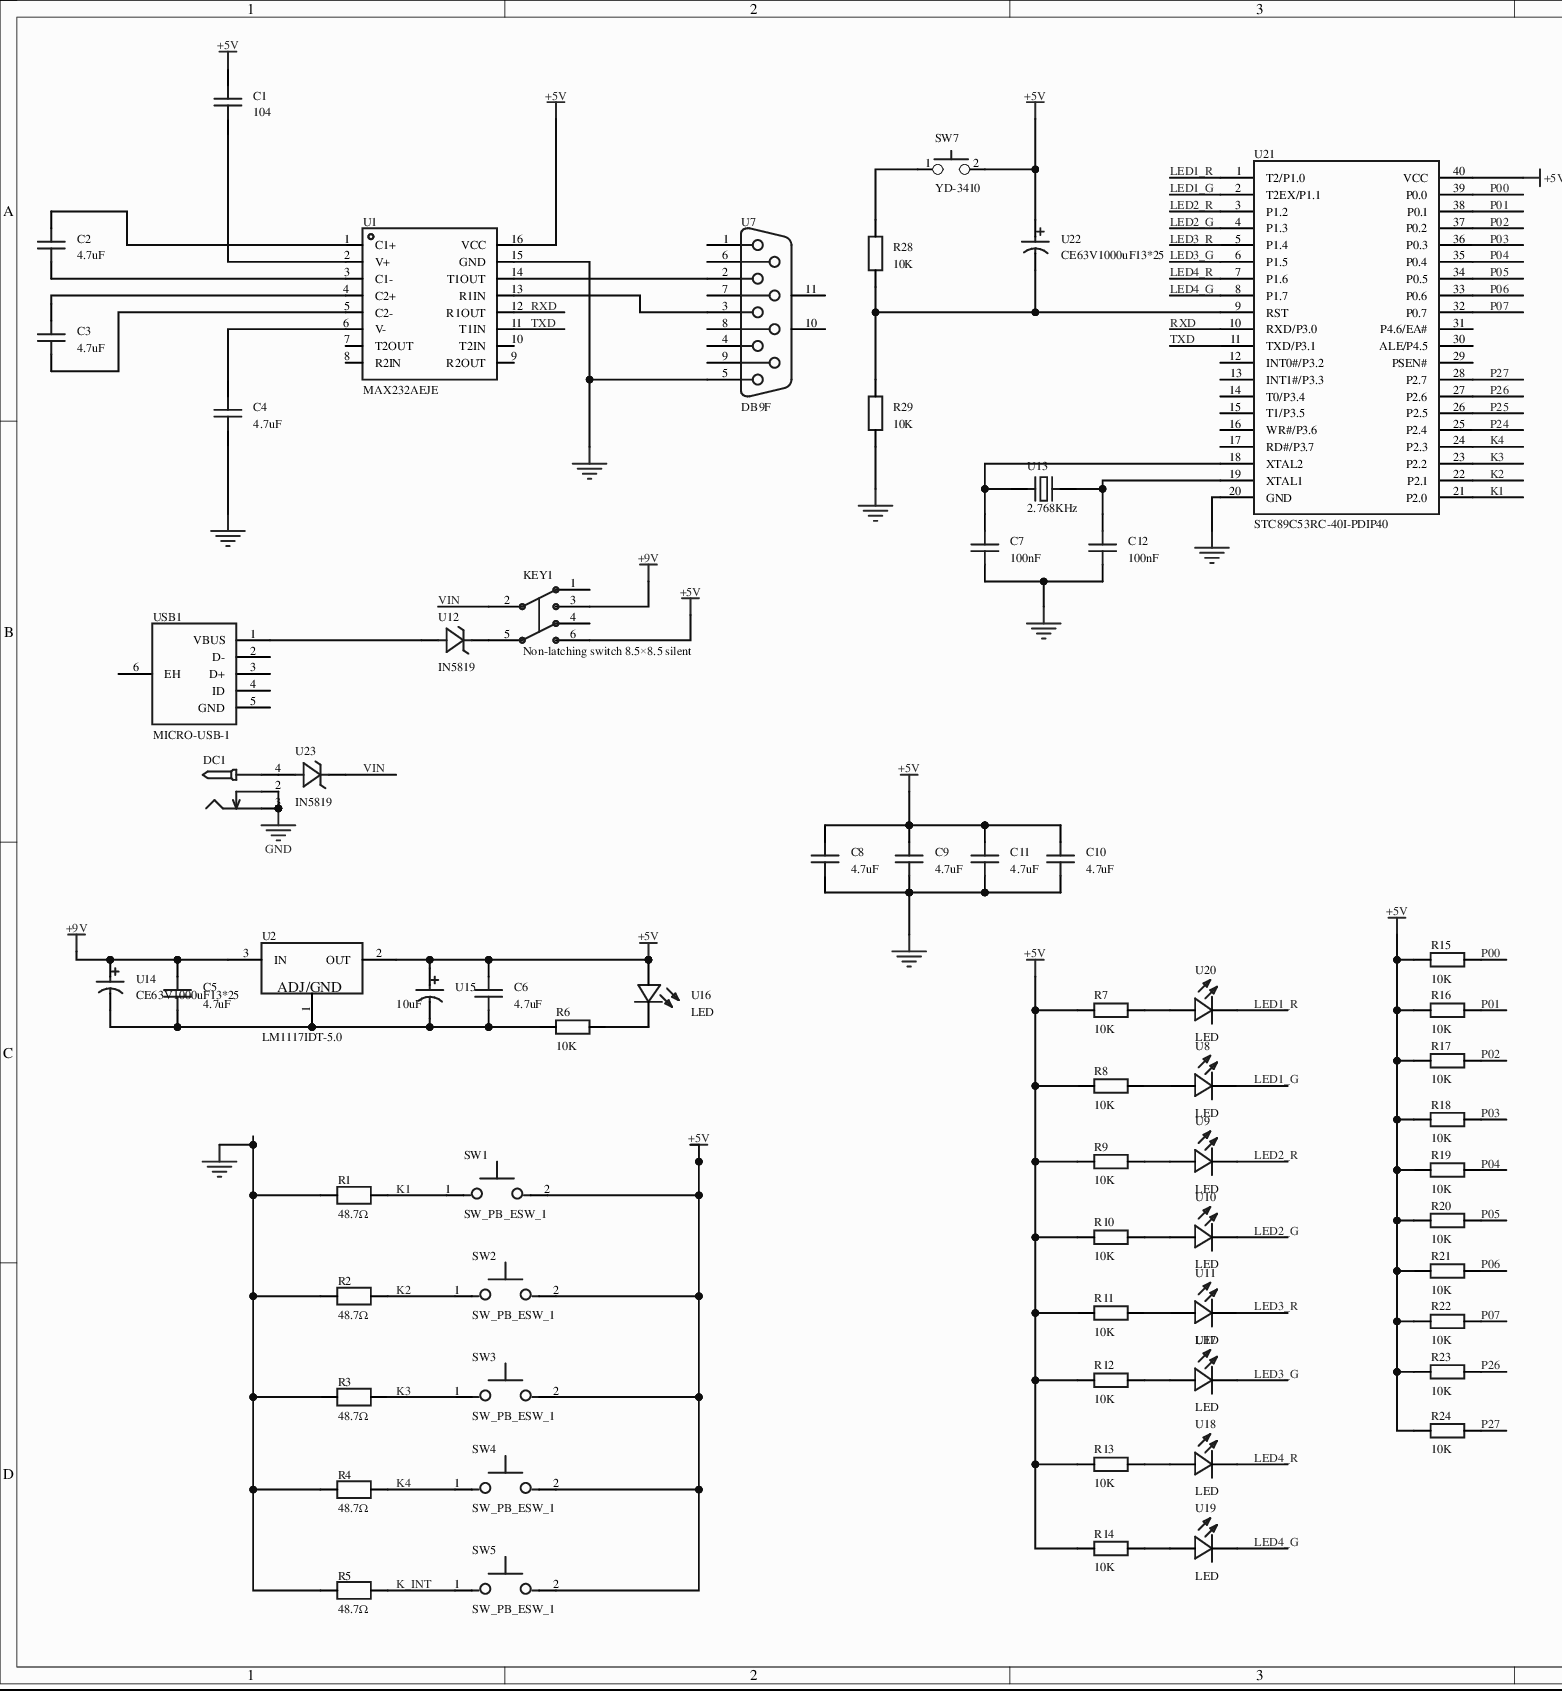
[diagram p0: MISC51895-3.schdoc, left]
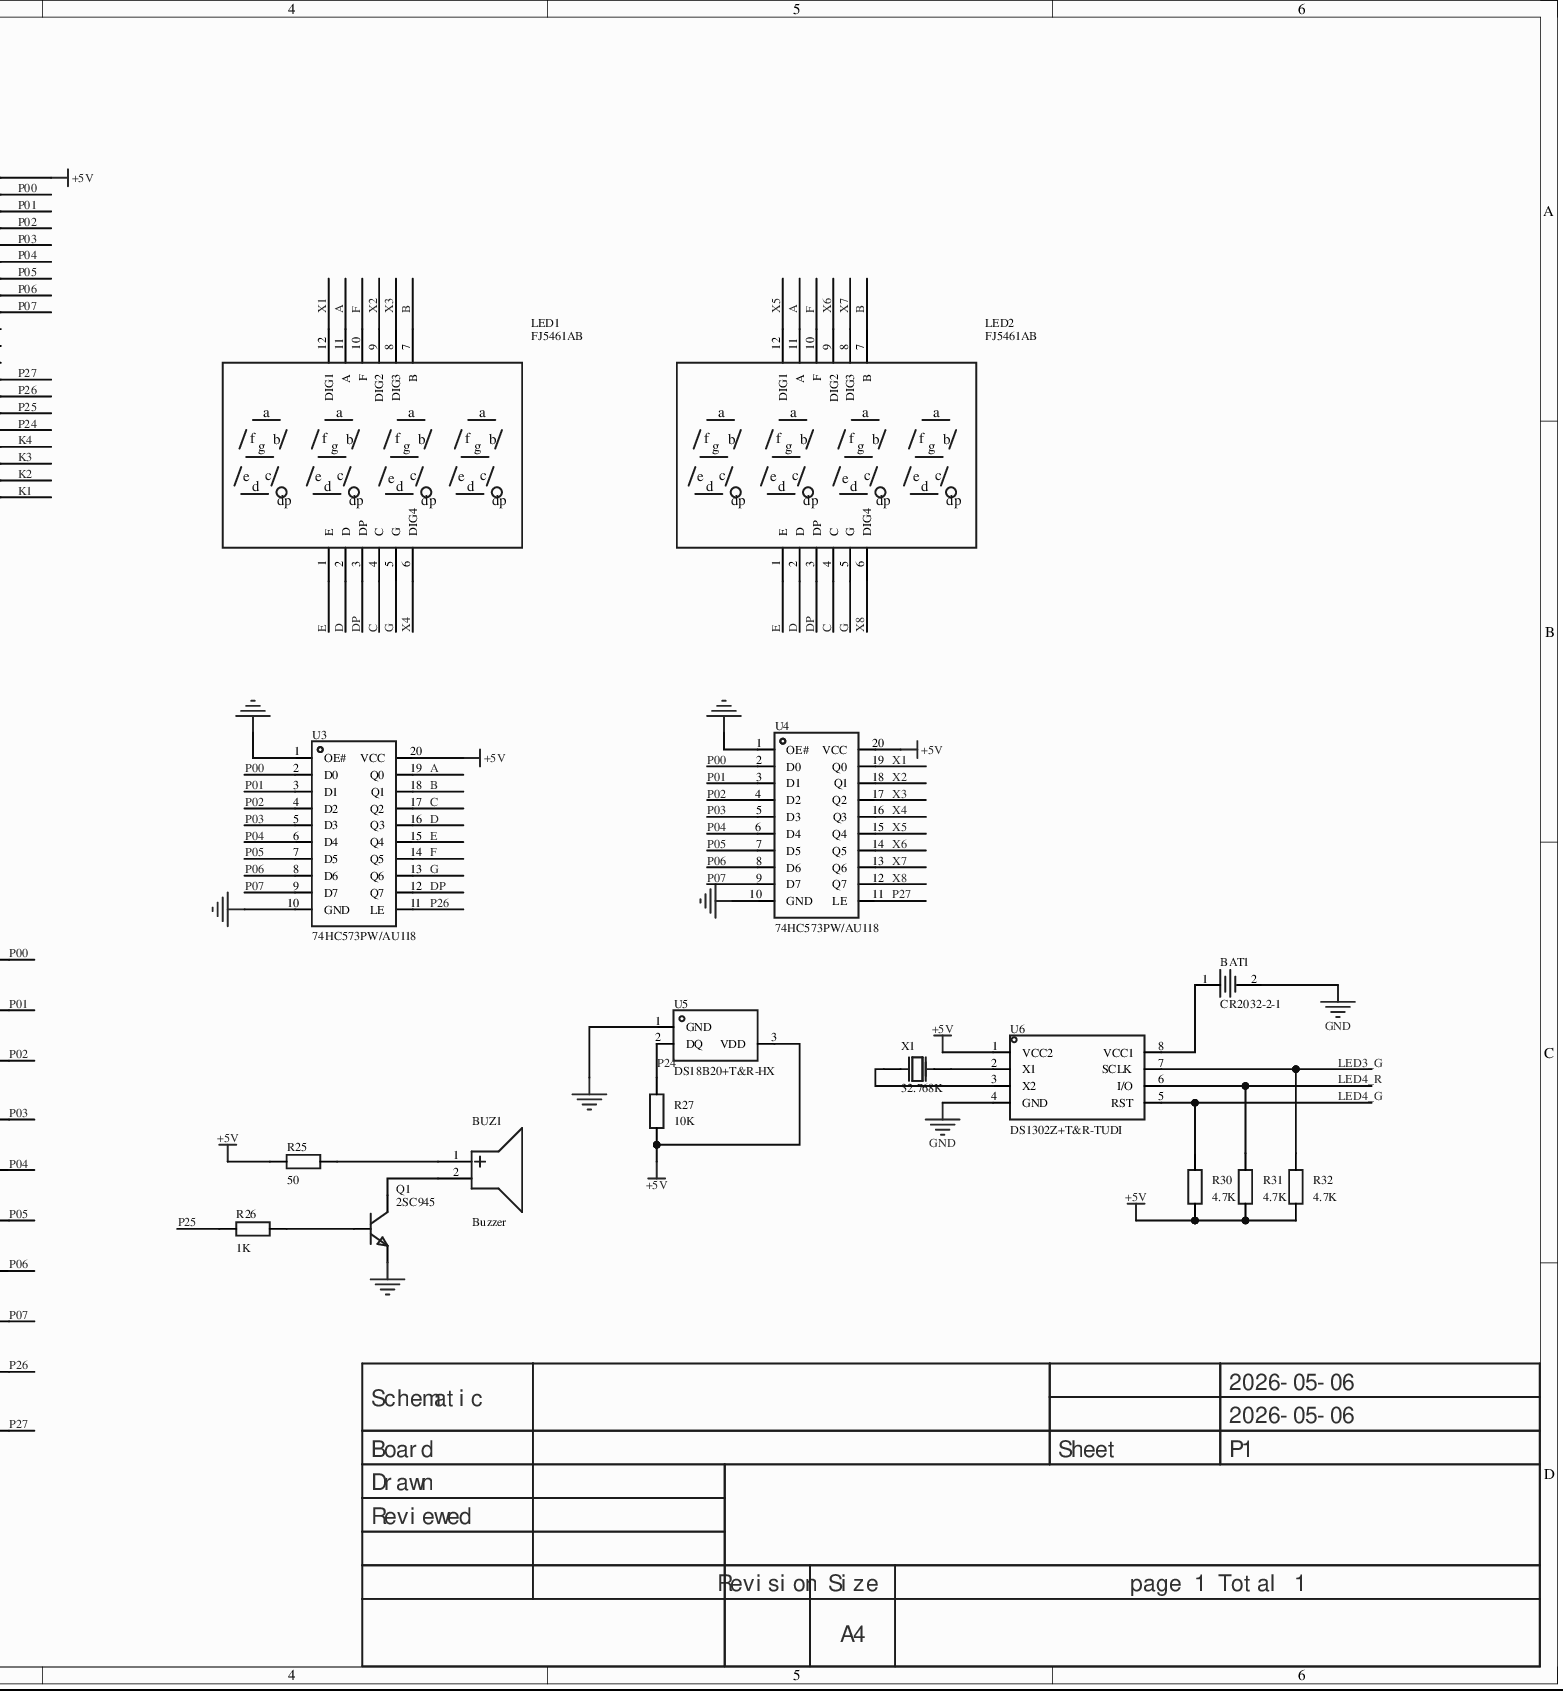
[diagram p1: MISC51895-3.schdoc, right]
# Altium project MISC51895-2.PrjPcb
1 sheet, 82 parts. Net scope: global (net labels, ports and power ports of the same name join across sheets).
Board file: MISC51895.pcbdoc

## Sheet MISC51895-3.schdoc
size 457 x 254 mm; Version: V1.0; @Project Name: MISC51895; @Update Date: 2026-05-06; @Create Date: 2026-05-06; @Board Name: MISC51895; @Create Time: 08:32:17; @Page Count: 1; @Page No: 1; @Schematic Name: MISC51895; @Update Time: 08:32:17; Size: A4

### Parts
BAT1  CR2032-2-1  [BAT-TH_CR2032-2-1]
BUZ1  Buzzer  [BUZ-TH_BD9.0-P5.00-D0.6-FD]
C1  104  [C0603]
C2  4.7uF  [C0603]
C3  4.7uF  [C0603]
C4  4.7uF  [C0603]
C5  4.7uF  [C0603]
C6  4.7uF  [C0603]
C7  100nF  [C0603]
C8  4.7uF  [C0603]
C9  4.7uF  [C0603]
C10  4.7uF  [C0603]
C11  4.7uF  [C0603]
C12  100nF  [C0603]
DC1  (no value)  [DC-2.0]
KEY1  Non-latching switch 8.5×8.5 silent  [SW-TH_6P-L8.5-W8.5-P2.54]
LED1  FJ5461AB  [LED-SEG-TH_12P-L50.4-W19.0-P2.54-S15.24-BL]
LED2  FJ5461AB  [LED-SEG-TH_12P-L50.4-W19.0-P2.54-S15.24-BL]
Q1  2SC945  [TO-92-3_L4.9-W3.7-P1.27-L]
R1  48.7Ω  [R0603]
R2  48.7Ω  [R0603]
R3  48.7Ω  [R0603]
R4  48.7Ω  [R0603]
R5  48.7Ω  [R0603]
R6  10K  [R0603]
R7  10K  [R0603]
R8  10K  [R0603]
R9  10K  [R0603]
R10  10K  [R0603]
R11  10K  [R0603]
R12  10K  [R0603]
R13  10K  [R0603]
R14  10K  [R0603]
R15  10K  [R0603]
R16  10K  [R0603]
R17  10K  [R0603]
R18  10K  [R0603]
R19  10K  [R0603]
R20  10K  [R0603]
R21  10K  [R0603]
R22  10K  [R0603]
R23  10K  [R0603]
R24  10K  [R0603]
R25  50  [R0603]
R26  1K  [R0603]
R27  10K  [R0603]
R28  10K  [R0603]
R29  10K  [R0603]
R30  4.7K  [R0603]
R31  4.7K  [R0603]
R32  4.7K  [R0603]
SW1  SW_PB_ESW_1  [KEY-SMD_L6.1-W3.8-LS8.0]
SW2  SW_PB_ESW_1  [KEY-SMD_L6.1-W3.8-LS8.0]
SW3  SW_PB_ESW_1  [KEY-SMD_L6.1-W3.8-LS8.0]
SW4  SW_PB_ESW_1  [KEY-SMD_L6.1-W3.8-LS8.0]
SW5  SW_PB_ESW_1  [KEY-SMD_L6.1-W3.8-LS8.0]
SW7  YD-3410  [SW-SMD_L3.9-W2.9-LS4.8-EH-A]
U1  MAX232AEJE  [PDIP-16_L19.3-W6.5-P2.54-LS7.6-BL]
U2  LM1117IDT-5.0  [TO-252-2_L6.6-W6.1-P4.57-LS9.7-BR-CW]
U3  74HC573PW/AU118  [TSSOP-20_L6.5-W4.4-P0.65-LS6.4-BL]
U4  74HC573PW/AU118  [TSSOP-20_L6.5-W4.4-P0.65-LS6.4-BL]
U5  DS18B20+T&R-HX  [TO-92-3_L5.1-W4.1-P1.27-L-1]
U6  DS1302Z+T&R-TUDI  [SOIC-8_L4.9-W3.9-P1.27-LS6.0-BL]
U7  DB9F  [DB9-TH_DB9F_C9900018961]
U8  LED  [LED-TH_BD4.0-P2.54-FD_RED]
U9  LED  [LED-TH_BD4.0-P2.54-FD_RED]
U10  LED  [LED-TH_BD4.0-P2.54-FD_RED]
U11  LED  [LED-TH_BD4.0-P2.54-FD_RED]
U12  IN5819  [SOD-123_L2.7-W1.7-LS3.8-RD]
U13  2.768KHz  [CRYSTAL-SMD_L3.2-W1.5-1]
U14  CE63V1000uF13*25  [CAP-TH_BD13.0-P5.00-D0.6-FD]
U15  10uF  [CAP-TH_BD13.0-P5.00-D0.6-FD]
U16  LED  [LED-TH_BD4.0-P2.54-FD_RED]
U17  LED  [LED-TH_BD4.0-P2.54-FD_RED]
U18  LED  [LED-TH_BD4.0-P2.54-FD_RED]
U19  LED  [LED-TH_BD4.0-P2.54-FD_RED]
U20  LED  [LED-TH_BD4.0-P2.54-FD_RED]
U21  STC89C53RC-40I-PDIP40  [DIP-40_L52.0-W13.7-P2.54-LS15.2-BL]
U22  CE63V1000uF13*25  [CAP-TH_BD13.0-P5.00-D0.6-FD]
U23  IN5819  [SOD-123_L2.7-W1.7-LS3.8-RD]
USB1  MICRO-USB-1  [MICRO-USB-SMD_C9900008946]
X1  32.768K  [OSC-SMD_L2.0-W1.2]

### Nets
+5V: C1.2 C6.2 C8.2 C9.2 C10.2 C11.2 KEY1.6 R7.1 R8.1 R9.1 R10.1 R11.1 R12.1 R13.1 R14.1 R15.1 R16.1 R17.1 R18.1 R19.1 R20.1 R21.1 R22.1 R23.1 R24.1 R25.1 R27.1 R30.1 R31.1 R32.1 SW1.2 SW2.2 SW3.2 SW4.2 SW5.2 SW7.2 U1.16(VCC) U2.2(OUT) U3.20(VCC) U4.20(VCC) U5.3(VDD) U6.1(VCC2) U15.1 U16.1(+) U21.40(VCC) U22.1
+9V: C5.2 KEY1.3 U2.3(IN) U14.1
GND: BAT1.2 C4.1 C7.1 C8.1 C9.1 C10.1 C11.1 C12.1 DC1.2 DC1.3 Q1.1(E) R1.1 R2.1 R3.1 R4.1 R5.1 R29.1 U1.15(GND) U3.1(OE#) U3.10(GND) U4.1(OE#) U4.10(GND) U5.1(GND) U6.4(GND) U7.5 U21.20(GND)
A: LED1.11(A) LED2.11(A) U3.19(Q0)
B: LED1.7(B) LED2.7(B) U3.18(Q1)
C: LED1.4(C) LED2.4(C) U3.17(Q2)
D: LED1.2(D) LED2.2(D) U3.16(Q3)
DP: LED1.3(DP) LED2.3(DP) U3.12(Q7)
E: LED1.1(E) LED2.1(E) U3.15(Q4)
F: LED1.10(F) LED2.10(F) U3.14(Q5)
G: LED1.5(G) LED2.5(G) U3.13(Q6)
K1: R1.2 SW1.1 U21.21(P2.0)
K2: R2.2 SW2.1 U21.22(P2.1)
K3: R3.2 SW3.1 U21.23(P2.2)
K4: R4.2 SW4.1 U21.24(P2.3)
K_INT: R5.2 SW5.1
LED1_G: U8.2(-) U21.2(T2EX/P1.1)
LED1_R: U20.2(-) U21.1(T2/P1.0)
LED2_G: U10.2(-) U21.4(P1.3)
LED2_R: U9.2(-) U21.3(P1.2)
LED3_G: R32.2 U6.7(SCLK) U17.2(-) U21.6(P1.5)
LED3_R: U11.2(-) U21.5(P1.4)
LED4_G: R30.2 U6.5(RST) U19.2(-) U21.8(P1.7)
LED4_R: R31.2 U6.6(I/O) U18.2(-) U21.7(P1.6)
P00: R15.2 U3.2(D0) U4.2(D0) U21.39(P0.0)
P01: R16.2 U3.3(D1) U4.3(D1) U21.38(P0.1)
P02: R17.2 U3.4(D2) U4.4(D2) U21.37(P0.2)
P03: R18.2 U3.5(D3) U4.5(D3) U21.36(P0.3)
P04: R19.2 U3.6(D4) U4.6(D4) U21.35(P0.4)
P05: R20.2 U3.7(D5) U4.7(D5) U21.34(P0.5)
P06: R21.2 U3.8(D6) U4.8(D6) U21.33(P0.6)
P07: R22.2 U3.9(D7) U4.9(D7) U21.32(P0.7)
P24: R27.2 U5.2(DQ) U21.25(P2.4)
P25: R26.1 U21.26(P2.5)
P26: R23.2 U3.11(LE) U21.27(P2.6)
P27: R24.2 U4.11(LE) U21.28(P2.7)
RXD: U1.12(R1OUT) U21.10(RXD/P3.0)
TXD: U1.11(T1IN) U21.11(TXD/P3.1)
VIN: KEY1.2 U23.1(K)
X1: LED1.12(DIG1) U4.19(Q0)
X2: LED1.9(DIG2) U4.18(Q1)
X3: LED1.8(DIG3) U4.17(Q2)
X4: LED1.6(DIG4) U4.16(Q3)
X5: LED2.12(DIG1) U4.15(Q4)
X6: LED2.9(DIG2) U4.14(Q5)
X7: LED2.8(DIG3) U4.13(Q6)
X8: LED2.6(DIG4) U4.12(Q7)
NetBAT1_1: BAT1.1 U6.8(VCC1)
NetBUZ1_1: BUZ1.1(+) R25.2
NetBUZ1_2: BUZ1.2(-) Q1.2(C)
NetC1_1: C1.1 U1.2(V+)
NetC2_1: C2.1 U1.3(C1-)
NetC2_2: C2.2 U1.1(C1+)
NetC3_1: C3.1 U1.5(C2-)
NetC3_2: C3.2 U1.4(C2+)
NetC4_2: C4.2 U1.6(V-)
NetC5_1: C5.1 C6.1 R6.1 U2.1(ADJ/GND) U14.2 U15.2
NetC7_2: C7.2 U13.1 U21.18(XTAL2)
NetC12_2: C12.2 U13.2 U21.19(XTAL1)
NetDC1_4: DC1.4 U23.2(A)
NetKEY1_5: KEY1.5 U12.1(K)
NetQ1_3: Q1.3(B) R26.2
NetR6_2: R6.2 U16.2(-)
NetR7_2: R7.2 U20.1(+)
NetR8_2: R8.2 U8.1(+)
NetR9_2: R9.2 U9.1(+)
NetR10_2: R10.2 U10.1(+)
NetR11_2: R11.2 U11.1(+)
NetR12_2: R12.2 U17.1(+)
NetR13_2: R13.2 U18.1(+)
NetR14_2: R14.2 U19.1(+)
NetR28_1: R28.1 R29.2 U21.9(RST) U22.2
NetR28_2: R28.2 SW7.1
NetU1_13: U1.13(R1IN) U7.3
NetU1_14: U1.14(T1OUT) U7.2
NetU6_2: U6.2(X1) X1.2(OSC2)
NetU6_3: U6.3(X2) X1.1(OSC1)
NetU12_2: U12.2(A) USB1.1(VBUS)

Not connected (* = marked no-connect by the designer): KEY1 1 4; U1 7(T2OUT) 8(R2IN) 9(R2OUT) 10(T2IN); U7 1 4 6 7 8 9 10(MH1) 11(MH2); U21 12(INT0#/P3.2) 13(INT1#/P3.3) 14(T0/P3.4) 15(T1/P3.5) 16(WR#/P3.6) 17(RD#/P3.7) 29(PSEN#) 30(ALE/P4.5) 31(P4.6/EA#); USB1 2(D-) 3(D+) 4(ID) 5(GND) 6(EH)

### Notes on the sheet
- 2026-05-06
- Schematic
- Board
- Sheet
- P1
- Drawn
- Reviewed
- Revision
- Size
- A4
- page 1 Total 1

### Library data of the parts
BAT1 = CR2032-2-1: AddInBom: yes; ModelId: 9f297eb2328241df835384c32afd7d320819f05c4eef4c71ace90d822a990e87; ModelTransform: 964.565,870.04,0,0,0,0,-42.047,0,-137.795; Symbol: CR2032-2-1; Device: CR2032-2-1; LCSC Part Name: CR2032-2-1; SupplierPart: C9900018737; ManufacturerPart: CR2032-2-1; Supplier Footprint: BATTERY_CR2032-A; JLCPCB Part Class: Extended Part; Supplier: LCSC; ConvertToPcb: yes; FootprintName: BAT-TH_CR2032-2-1; ModelName: BAT-TH_CR2032-2-1
BUZ1 = 蜂鸣器: AddInBom: yes; ModelId: 13273335caac486e928bafb4d9fdf12d0819f05c4eef4c71ace90d822a990e87; ModelName: BUZ-TH_D9.0-H5.5-P5.0; ModelTransform: 354.33,354.33,0,90,0,0,-0.005,0,-177.165; Symbol: Buzzer; Device: Buzzer; LCSC Part Name: 蜂鸣器; SupplierPart: C9900020875; ManufacturerPart: 蜂鸣器; Supplier Footprint: 插件; JLCPCB Part Class: Extended Part; Supplier: LCSC; ConvertToPcb: yes; FootprintName: BUZ-TH_BD9.0-P5.00-D0.6-FD
C1-C6 C8-C11 = GRM188R61A475KAAJD: Capacitance: 4.7uF; tolerance: ±10%; rated voltage: 10V; temperature coefficient: X5R;; Manufacturer: muRata(村田); AddInBom: yes; ModelId: ac125912035d415993ca9572d50418b10819f05c4eef4c71ace90d822a990e87; ModelName: C0603_L1.6-W0.8-H0.8; ModelTransform: 62.992,31.496,0,0,0,0,0,0,0; Symbol: GRM188R61A475KAAJD; Device: GRM188R61A475KAAJD; LCSC Part Name: 4.7uF ±10% 10V; ManufacturerPart: GRM188R61A475KAAJD; Supplier Footprint: 0603; JLCPCB Part Class: Extended Part; Supplier: LCSC; ConvertToPcb: yes; FootprintName: C0603; Tolerance: ±10%; Voltage Rating: 10V; Temperature Coefficient: X5R
  C1: Value: 104
  C2-C6 C8-C11: SupplierPart: C668355; Value: 4.7uF
C7 C12 = CAP_0603: Symbol: Capacitance; ConvertToPcb: yes; ModelId: ac125912035d415993ca9572d50418b10819f05c4eef4c71ace90d822a990e87; ModelName: C0603_L1.6-W0.8-H0.8; ModelTransform: 62.992,31.496,0,0,0,0,0,0,0; Device: CAP_0603; AddInBom: yes; Supplier Footprint: 0603; FootprintName: C0603; Value: 100nF
DC1 = DC-005_2.0: Symbol: DC power jack; ConvertToPcb: yes; ModelId: f5f20b8a2308479b936ba3c2698865bb0819f05c4eef4c71ace90d822a990e87; ModelName: DC-IN-TH_DC-5520-1; ModelTransform: 372.05,551.18,582.68,90,0,0,137.8,0,-149.61; Device: DC-005_2.0; AddInBom: yes; Supplier Footprint: 插件; FootprintName: DC-2.0
KEY1 = 无自锁开关 8.5×8.5 无声: 6 pins, 8.5×8.5; Symbol: No self-locking switch 8.5×8.5 silent; AddInBom: yes; ModelId: 4c72b3966b92446eb355e1bd0fb4f8800819f05c4eef4c71ace90d822a990e87; ModelTransform: 342.519,334.645,0,180,0,0,0,0,-137.795; Device: Non-latching switch 8.5×8.5 silent; LCSC Part Name: 无自锁开关 8.5×8.5  无声; SupplierPart: C26228; ManufacturerPart: 无自锁开关 8.5×8.5 无声; Supplier Footprint: 插件; JLCPCB Part Class: Extended Part; Supplier: LCSC; ConvertToPcb: yes; FootprintName: SW-TH_6P-L8.5-W8.5-P2.54; ModelName: SW-TH_6P-L8.5-W8.5-P2.54
LED1 LED2 = FJ5461AB: AddInBom: yes; ModelId: 9ac57c94fd454ea28a76cabfc3090fc50819f05c4eef4c71ace90d822a990e87; ModelTransform: 1984.248,748.424,0,0,0,0,0,-1.969,-196.85; Symbol: FJ5461AB; Device: FJ5461AB; LCSC Part Name: FJ5461AB; SupplierPart: C9900022126; ManufacturerPart: FJ5461AB; Supplier Footprint: SMG0.56-4P; JLCPCB Part Class: Extended Part; Supplier: LCSC; ConvertToPcb: yes; FootprintName: LED-SEG-TH_12P-L50.4-W19.0-P2.54-S15.24-BL; ModelName: LED-SEG-TH_12P-L50.4-W19.0-P2.54-S15.24-BL
Q1 = 2SC945: Manufacturer: ST(先科); Symbol: 2SC945_C2987754; AddInBom: yes; ModelId: aafe8e06f2154e7c93506efd0d6632dd0819f05c4eef4c71ace90d822a990e87; ModelTransform: 176.28752,144.88554,0,180,0,0,0,20.669,-196.85; Device: 2SC945; LCSC Part Name: 三极管 停产; SupplierPart: C2987754; ManufacturerPart: 2SC945; Supplier Footprint: TO-92-3; JLCPCB Part Class: Extended Part; Datasheet: example.com/20220401/866B6C811E060AF67E1650FE9BEED438.pdf; Supplier: LCSC; ConvertToPcb: yes; FootprintName: TO-92-3_L4.9-W3.7-P1.27-L; ModelName: TO-92-3_L4.9-W3.7-P1.27-L
R1-R5 = FRC0603F48R7TS: Resistor type: thick film resistor; resistance: 48.7Ω; tolerance: ±1%; power: 100mW; working voltage: 75V; temperature coefficient: ±100ppm/℃;; Manufacturer: FOJAN(富捷); AddInBom: yes; ModelId: fc143cca1e79419f9cd78b61e9279f080819f05c4eef4c71ace90d822a990e87; ModelTransform: 31.8897,63.7794,0,90,0,0,0,0,0; Symbol: FRC0603F48R7TS; Device: FRC0603F48R7TS; LCSC Part Name: 厚膜电阻 48.7Ω ±1% 100mW; SupplierPart: C51048260; ManufacturerPart: FRC0603F48R7TS; Supplier Footprint: 0603; JLCPCB Part Class: Extended Part; Supplier: LCSC; ConvertToPcb: yes; FootprintName: R0603; ModelName: R0603; Type: Thick film resistor; Value: 48.7Ω; Tolerance: ±1%; Power(Watts): 100mW; Voltage-Supply(Max): 75V; Temperature Coefficient: ±100ppm/℃; Operating Temperature: -55℃~+155℃
R6-R29 = Res_0603: Symbol: Resistor; ConvertToPcb: yes; ModelId: fc143cca1e79419f9cd78b61e9279f080819f05c4eef4c71ace90d822a990e87; ModelTransform: 31.8897,63.7794,0,90,0,0,0,0,0; Device: Res_0603; AddInBom: yes; Supplier Footprint: 0603; FootprintName: R0603; ModelName: R0603
  R6-R24 R27-R29: Value: 10K
  R25: Value: 50
  R26: Value: 1K
R30-R32 = Res_0603: Symbol: Resistor; 3D Model: fc143cca1e79419f9cd78b61e9279f080819f05c4eef4c71ace90d822a990e87; 3D Model Transform: 31.8897,63.7794,0,90,0,0,0,0,0; ConvertToPcb: yes; Device: Res_0603; Supplier Footprint: 0603; Value: 4.7K; AddInBom: yes; FootprintName: R0603; ModelName: R0603
SW1-SW5 = SW_PB_ESW_1: AddInBom: yes; ModelId: 34031407cd58403392f505751e0e661e0819f05c4eef4c71ace90d822a990e87; ModelTransform: 314.96,149.606,0,0,0,0,0,0,0; Symbol: SW_PB_ESW_1; Device: SW_PB_ESW_1; LCSC Part Name: SW_PB_ESW_1; SupplierPart: C9900009156; ManufacturerPart: SW_PB_ESW_1; Supplier Footprint: SW_PB_ESW_1; JLCPCB Part Class: Extended Part; Supplier: LCSC; ConvertToPcb: yes; FootprintName: KEY-SMD_L6.1-W3.8-LS8.0; ModelName: KEY-SMD_L6.1-W3.8-LS8.0
SW7 = YD-3410: AddInBom: yes; Symbol: YD-3410; Device: YD-3410; LCSC Part Name: YD-3410; SupplierPart: C9900006416; ManufacturerPart: YD-3410; Supplier Footprint: SW-PB; JLCPCB Part Class: Extended Part; Supplier: LCSC; ConvertToPcb: yes; FootprintName: SW-SMD_L3.9-W2.9-LS4.8-EH-A
U1 = MAX232AEJE: Type: transceiver; data rate: 120Kbps;; Manufacturer: ADI(亚德诺)/MAXIM(美信); AddInBom: yes; ModelId: fbf64f1066904807ba848675b6d2e65d0819f05c4eef4c71ace90d822a990e87; ModelName: PDIP-16_L19.3-W6.5-H5.1-P2.54-LS7.6-BL; ModelTransform: 787.4,311.8104,0,0,0,0,0,0,-118.11; Number of Driver: 2; Supply Voltage: 4.5V~5.5V; Symbol: MAX232AEJE; Device: MAX232AEJE; LCSC Part Name: MAX232AEJE; SupplierPart: C3214045; ManufacturerPart: MAX232AEJE; Supplier Footprint: CDIP-16; JLCPCB Part Class: Extended Part; Datasheet: example.com/20180126/C143394_15169558667671308916.pdf; Supplier: LCSC; ConvertToPcb: yes; FootprintName: PDIP-16_L19.3-W6.5-P2.54-LS7.6-BL; Types: Transceiver; Number of receiver: 2; Data Rate: 120Kbps; Operating Temperature: -40℃~+85℃
U2 = LM1117IDT-5.0: Output type: fixed; max input voltage: 15V; output voltage: 5V; max output current: 800mA; PSRR: 75dB@(120Hz); output polarity: positive;; Manufacturer: TI(德州仪器); AddInBom: yes; ModelId: b25cb2d73e164a43b9271668fe9a6fe30819f05c4eef4c71ace90d822a990e87; ModelTransform: 381.889,264.58774,0,0,0,0,-42.323,0,0; Dropout Voltage: 1.2V@(800mA); standby current: 5mA; Number of Outputs: 1; Symbol: LM1117IDT-5.0; Device: LM1117IDT-5.0; LCSC Part Name: LM1117IDT-5.0; SupplierPart: C3750736; ManufacturerPart: LM1117IDT-5.0; Supplier Footprint: TO-252-3; JLCPCB Part Class: Extended Part; Datasheet: example.com/20230925/18486D0921DA4BEFFA0AABA1603EA6DC.pdf; Supplier: LCSC; ConvertToPcb: yes; FootprintName: TO-252-2_L6.6-W6.1-P4.57-LS9.7-BR-CW; ModelName: TO-252-2_L6.6-W6.1-P4.57-LS9.7-BR-CW; Output Type: Fixed; Maximum Input Voltage: 15V; Output Voltage: 5V; MAX Output Current: 800mA; Power Supply Rejection Ratio (PSRR): 75dB@(120Hz); Operating Temperature: -40℃~+125℃; Output Polarity: Positive
U3 U4 = 74HC573PW/AU118: Manufacturer: Nexperia(安世); AddInBom: yes; ModelId: c491f68934b34c649df5890a1d97cd0f0819f05c4eef4c71ace90d822a990e87; ModelName: TSSOP-20_L6.5-W4.4-H1.0-LS6.4-P0.65; ModelTransform: 251.969,255.906,0,90,0,0,0.0005,0,0; Symbol: 74HC573PW/AU118; Device: 74HC573PW/AU118; LCSC Part Name: 74HC573PW/AU118; SupplierPart: C4989176; ManufacturerPart: 74HC573PW/AU118; Supplier Footprint: TSSOP-20; JLCPCB Part Class: Extended Part; Supplier: LCSC; ConvertToPcb: yes; FootprintName: TSSOP-20_L6.5-W4.4-P0.65-LS6.4-BL
U5 = DS18B20+T&R-HX: Detection temperature: -; accuracy: ±0.5℃; interface type: single-bus;; Manufacturer: ZHHXDZ(海芯电子); AddInBom: yes; ModelId: 3974197e164648709a3727be714795da0819f05c4eef4c71ace90d822a990e87; ModelTransform: 200.42283,161.417,0,0,0,0,0,9.842,-196.85; Voltage - Supply: 3V~5.5V; Standby Current: 500nA; Temperature Conversion Time: 500ms; Temperature Resolution: 12bit; Symbol: DS18B20+T&R-HX; Device: DS18B20+T&R-HX; LCSC Part Name: DS18B20+T&R-HX; SupplierPart: C52034466; ManufacturerPart: DS18B20+T&R-HX; Supplier Footprint: TO-92; JLCPCB Part Class: Extended Part; Supplier: LCSC; ConvertToPcb: yes; FootprintName: TO-92-3_L5.1-W4.1-P1.27-L-1; ModelName: TO-92-3_L5.1-W4.1-P1.27-L-1; Detection Temperature Range: -; Tolerance: ±0.5℃; Interface: single-bus; Operating Temperature: -
U6 = DS1302Z+T&R-TUDI: Real-time clock (RTC); Manufacturer: TD(钍地半导体); AddInBom: yes; ModelId: e81d2f7d937b4a6ab1dca543ff5d56a40819f05c4eef4c71ace90d822a990e87; ModelName: SOIC-8_L4.9-W3.9-H1.7-LS6.0-P1.27; ModelTransform: 192.913,236.22,0,0,0,0,0,0,0; Symbol: DS1302Z+T&R-TUDI; Device: DS1302Z+T&R-TUDI; LCSC Part Name: DS1302Z+T&R-TUDI; SupplierPart: C54741334; ManufacturerPart: DS1302Z+T&R-TUDI; Supplier Footprint: SOP-8; JLCPCB Part Class: Extended Part; Supplier: LCSC; ConvertToPcb: yes; FootprintName: SOIC-8_L4.9-W3.9-P1.27-LS6.0-BL
U7 = DB9F: AddInBom: yes; ModelId: ef06ade5e717490592459d28fa0205e80819f05c4eef4c71ace90d822a990e87; ModelTransform: 1212.596,716.57341,0,0,0,0,0,-242.126,-157.48; Symbol: DB9F; Device: DB9F; LCSC Part Name: DB9F; SupplierPart: C9900018961; ManufacturerPart: DB9F; Supplier Footprint: DB9; JLCPCB Part Class: Extended Part; Supplier: LCSC; ConvertToPcb: yes; FootprintName: DB9-TH_DB9F_C9900018961; ModelName: DB9-TH_DB9F_C9900018961
U8-U11 U16-U20 = LED: Symbol: LED_C9900015665; AddInBom: yes; ModelId: 08d245f9ade94e79a608b24242b3e8900819f05c4eef4c71ace90d822a990e87; ModelTransform: 137.561,157.46465,0,0,0,0,-8.858,0,-196.85; Device: LED; LCSC Part Name: LED; SupplierPart: C9900015665; ManufacturerPart: LED; Supplier Footprint: SIP-2P; JLCPCB Part Class: Extended Part; Supplier: LCSC; ConvertToPcb: yes; FootprintName: LED-TH_BD4.0-P2.54-FD_RED; ModelName: LED-TH_BD4.0-P2.54-FD_RED
U12 = IN5819_C9900008333: AddInBom: yes; ModelId: b455d3bf1dad47d3a75f9a76b08071c60819f05c4eef4c71ace90d822a990e87; ModelTransform: 145.669,64.961,0,0,0,0,0,0,0; Symbol: IN5819_C9900008333; Device: IN5819_C9900008333; LCSC Part Name: IN5819; SupplierPart: C9900008333; ManufacturerPart: IN5819; Supplier Footprint: SOD-123; JLCPCB Part Class: Extended Part; Supplier: LCSC; ConvertToPcb: yes; FootprintName: SOD-123_L2.7-W1.7-LS3.8-RD; ModelName: SOD-123_L2.7-W1.7-LS3.8-RD
U13 = 2.768KHz: AddInBom: yes; ModelId: 762d7afc596f4558a373612390f4386d0819f05c4eef4c71ace90d822a990e87; ModelTransform: 125.984,59.055,0,0,0,0,0,0,0; Symbol: 2.768KHZ; Device: 2.768KHz; LCSC Part Name: 2.768KHz; SupplierPart: C9900022434; ManufacturerPart: 2.768KHz; Supplier Footprint: CRYSTAL_2PIN; JLCPCB Part Class: Extended Part; Supplier: LCSC; ConvertToPcb: yes; FootprintName: CRYSTAL-SMD_L3.2-W1.5-1; ModelName: CRYSTAL-SMD_L3.2-W1.5-1
U14 U15 U22 = CE63V1000uF13*25: AddInBom: yes; ModelId: d480d9258dff471ebe4ee69eb07122f60819f05c4eef4c71ace90d822a990e87; ModelName: CAP-TH_BD13.0-P5.00-D1.2-FD; ModelTransform: 492.5187,492.025,0,0,0,0,-0.005,0,-137.795; Symbol: CE63V1000UF13*25; Device: CE63V1000uF13*25; LCSC Part Name: CE63V1000uF13*25; SupplierPart: C9900014985; Supplier Footprint: 电解电容13*25mm; JLCPCB Part Class: Extended Part; Supplier: LCSC; ConvertToPcb: yes; FootprintName: CAP-TH_BD13.0-P5.00-D0.6-FD
  U14 U22: ManufacturerPart: CE63V1000uF13*25
  U15: Manufacturer Part: 10uF
U21 = STC89C53RC-40I-PDIP40: CPU core: 51 family;; Manufacturer: STC; Symbol: STC89C53RC_C22295; AddInBom: yes; ModelId: 16d4686a009b4ddca948f91eddb57b140819f05c4eef4c71ace90d822a990e87; ModelName: DIP-40_L52.3-W13.8-H4.0-LS15.24-P2.54; ModelTransform: 2059.051,615.743,0,0,0,0,0,0,-118.11; Program Storage Size: 12KB; Program Memory Type: FLASH; Number of I/O: 35; Voltage - Supply: 3.5V~5.5V; Device: STC89C53RC-40I-PDIP40; LCSC Part Name: STC89C53RC-40I-PDIP40; SupplierPart: C22295; ManufacturerPart: STC89C53RC-40I-PDIP40; Supplier Footprint: DIP-40; JLCPCB Part Class: Extended Part; Supplier: LCSC; ConvertToPcb: yes; FootprintName: DIP-40_L52.0-W13.7-P2.54-LS15.2-BL; CPU Core: 51 family
U23 = IN5819_C9900008333: 3D Model: b455d3bf1dad47d3a75f9a76b08071c60819f05c4eef4c71ace90d822a990e87; 3D Model Transform: 145.669,64.961,0,0,0,0,0,0,0; AddInBom: yes; Symbol: IN5819_C9900008333; Device: IN5819_C9900008333; LCSC Part Name: IN5819; Supplier Part: C9900008333; Manufacturer Part: IN5819; Supplier Footprint: SOD-123; JLCPCB Part Class: Extended Part; Supplier: LCSC; ConvertToPcb: yes; FootprintName: SOD-123_L2.7-W1.7-LS3.8-RD; ModelName: SOD-123_L2.7-W1.7-LS3.8-RD
USB1 = MICRO-USB-1: AddInBom: yes; ModelId: 03278485a0ad4b6f9ea4a64b4dabf4cb0819f05c4eef4c71ace90d822a990e87; ModelTransform: 314.96,223.6216,0,0,0,0,0,-49.213,-39.37; Symbol: MICRO-USB-1; Device: MICRO-USB-1; LCSC Part Name: MICRO-USB-1; SupplierPart: C9900008946; ManufacturerPart: MICRO-USB-1; Supplier Footprint: USB-micro; JLCPCB Part Class: Extended Part; Supplier: LCSC; ConvertToPcb: yes; FootprintName: MICRO-USB-SMD_C9900008946; ModelName: MICRO-USB-SMD_C9900008946
X1 = 32.768K: AddInBom: yes; ModelId: cb5fefbe4132494b9adb268fbf3d1f9d0819f05c4eef4c71ace90d822a990e87; ModelName: OSC-SMD_L2.0-W1.2-H0.5; ModelTransform: 78.74,47.244,0,0,0,0,0,0,0; Symbol: 32.768K; Device: 32.768K; LCSC Part Name: 32.768K; SupplierPart: C9900010122; ManufacturerPart: 32.768K; Supplier Footprint: SMD2012-2P; JLCPCB Part Class: Extended Part; Supplier: LCSC; ConvertToPcb: yes; FootprintName: OSC-SMD_L2.0-W1.2